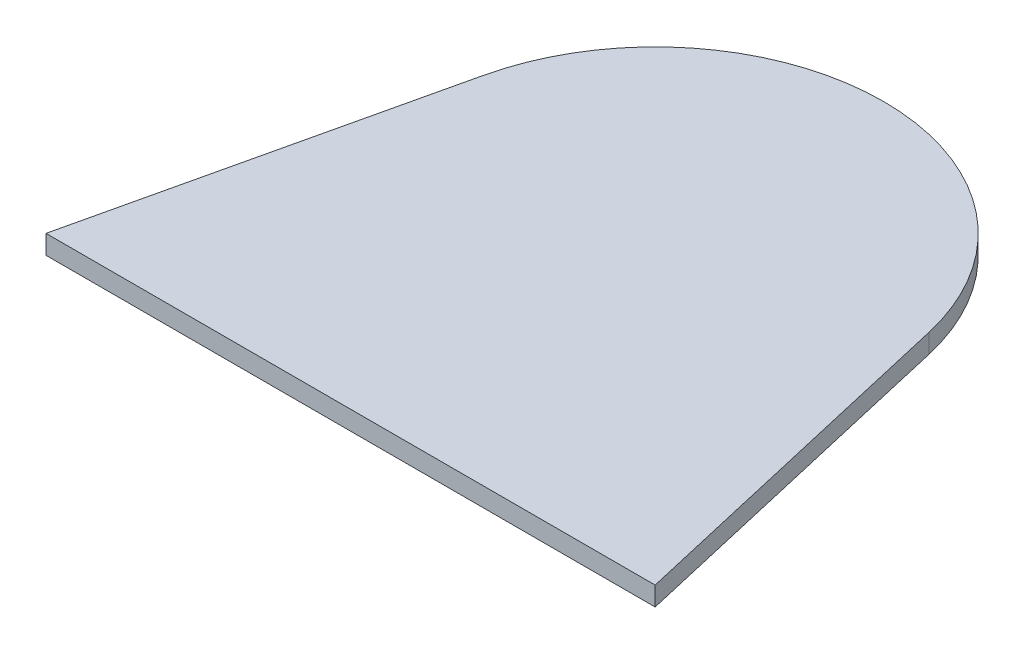
from build123d import *

# Parameters (mm, degrees)
EXTRUDE_1_DEPTH = 5


with BuildPart() as part:
    # 草图1 → 凸台-拉伸1 (new body)
    with BuildSketch(Plane(origin=(0, 0, 0), x_dir=(1, 0, 0), z_dir=(0, 1, 0))):
        with BuildLine():
            Line((80, -80), (-80, -80))
            Line((-80, -80), (-58.468736425, 13.468736425))
            ThreePointArc((-58.468736425, 13.468736425), (0, 60), (58.468736425, 13.468736425))
            Line((58.468736425, 13.468736425), (80, -80))
        make_face()
    extrude(amount=EXTRUDE_1_DEPTH)


solid = part.part
